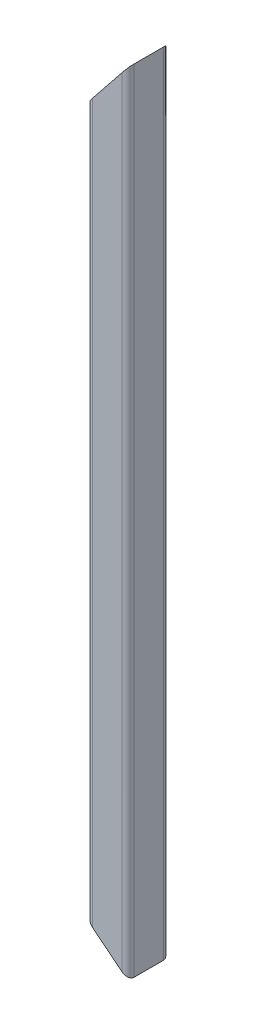
from build123d import *

# Parameters (mm, degrees)
F_19_WELDMEMBERFEAT_4_MORE_IN_5_FILES_DEPTH = 1340
CUT_EXTRUDE1_DEPTH                          = 1343.283502096
CUT_EXTRUDE1_DEPTH_BACK                     = 1343.283502096


with BuildPart() as part:
    # Sketch1 → 19 (WeldMemberFeat) (+4 more in 5 files) Cold-formed hollow square steel (GB/T 6728-2002) 70×70×5(1) (new body)
    with BuildSketch(Plane(origin=(0, 0, 0), x_dir=(-1, 0, 0), z_dir=(0, 1, 0))):
        with BuildLine():
            Line((-25, -35), (25, -35))
            ThreePointArc((25, -35), (32.071067812, -32.071067812), (35, -25))
            Line((35, -25), (35, 25))
            ThreePointArc((35, 25), (32.071067812, 32.071067812), (25, 35))
            Line((25, 35), (-25, 35))
            ThreePointArc((-25, 35), (-32.071067812, 32.071067812), (-35, 25))
            Line((-35, 25), (-35, -25))
            ThreePointArc((-35, -25), (-32.071067812, -32.071067812), (-25, -35))
        make_face()
        with BuildLine():
            Line((-25, -30), (25, -30))
            ThreePointArc((25, -30), (28.535533906, -28.535533906), (30, -25))
            Line((30, -25), (30, 25))
            ThreePointArc((30, 25), (28.535533906, 28.535533906), (25, 30))
            Line((25, 30), (-25, 30))
            ThreePointArc((-25, 30), (-28.535533906, 28.535533906), (-30, 25))
            Line((-30, 25), (-30, -25))
            ThreePointArc((-30, -25), (-28.535533906, -28.535533906), (-25, -30))
        make_face(mode=Mode.SUBTRACT)
    extrude(amount=F_19_WELDMEMBERFEAT_4_MORE_IN_5_FILES_DEPTH)

    # Sketch2 → Cut-Extrude1 (cut, two sides: drawn at the far end of the back side and taken through both)
    with BuildSketch(Plane.XY.offset(35).offset(-CUT_EXTRUDE1_DEPTH_BACK)):
        Polygon((35, 1340), (-35, 1252.5), (-35, 1340), align=None)
        Polygon((-35, 56), (35, 0), (-35, 0), align=None)
    extrude(amount=CUT_EXTRUDE1_DEPTH + CUT_EXTRUDE1_DEPTH_BACK, mode=Mode.SUBTRACT)


solid = part.part
